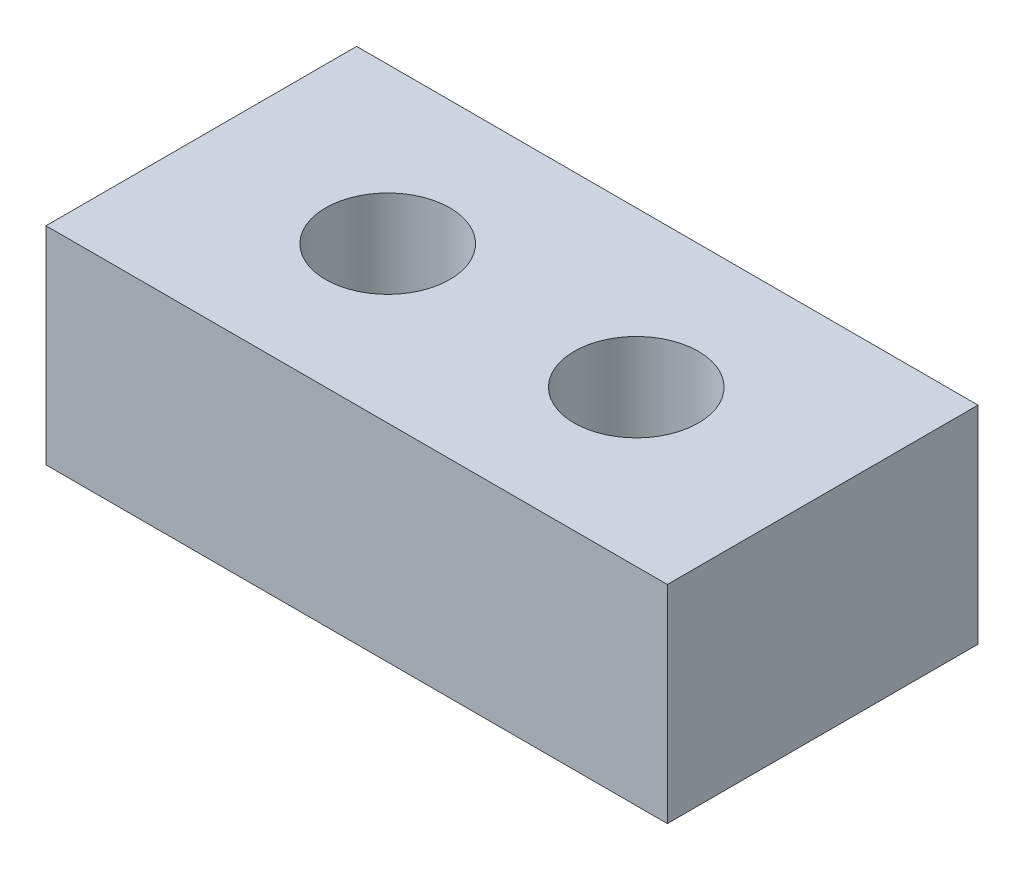
SolidWorks part; units mm, degrees
ref_plane "Front Plane" through (0, 0, 0) normal (0, 0, 1) x (1, 0, 0)
ref_plane "Top Plane" through (0, 0, 0) normal (0, 1, 0) x (1, 0, 0)
ref_plane "Right Plane" through (0, 0, 0) normal (1, 0, 0) x (0, 0, -1)
other "Configuration Table"
sketch "Sketch1" plane through (0, 0, 0) normal (0, 1, 0) x (1, 0, 0)
  line L1 (-150, 75) -> (150, 75)
  line L2 (-150, 75) -> (-150, -75)
  line L3 (-150, -75) -> (150, -75)
  line L4 (150, 75) -> (150, -75)
  line L5 (-150, 75) -> (150, -75) construction
  line L6 (-150, -75) -> (150, 75) construction
  circle A0 centre (60, 0) radius 30
  circle A1 centre (-60, 0) radius 30
  point P0 (0, 0)
  dimension "D3" = 60
  dimension "D4" = 60
  dimension "D6" = 90
  dimension "D1" = 150
  dimension "D2" = 300
  dimension "D5" = 90
extrude "Boss-Extrude1" add sketch "Sketch1" along normal mid plane 100
